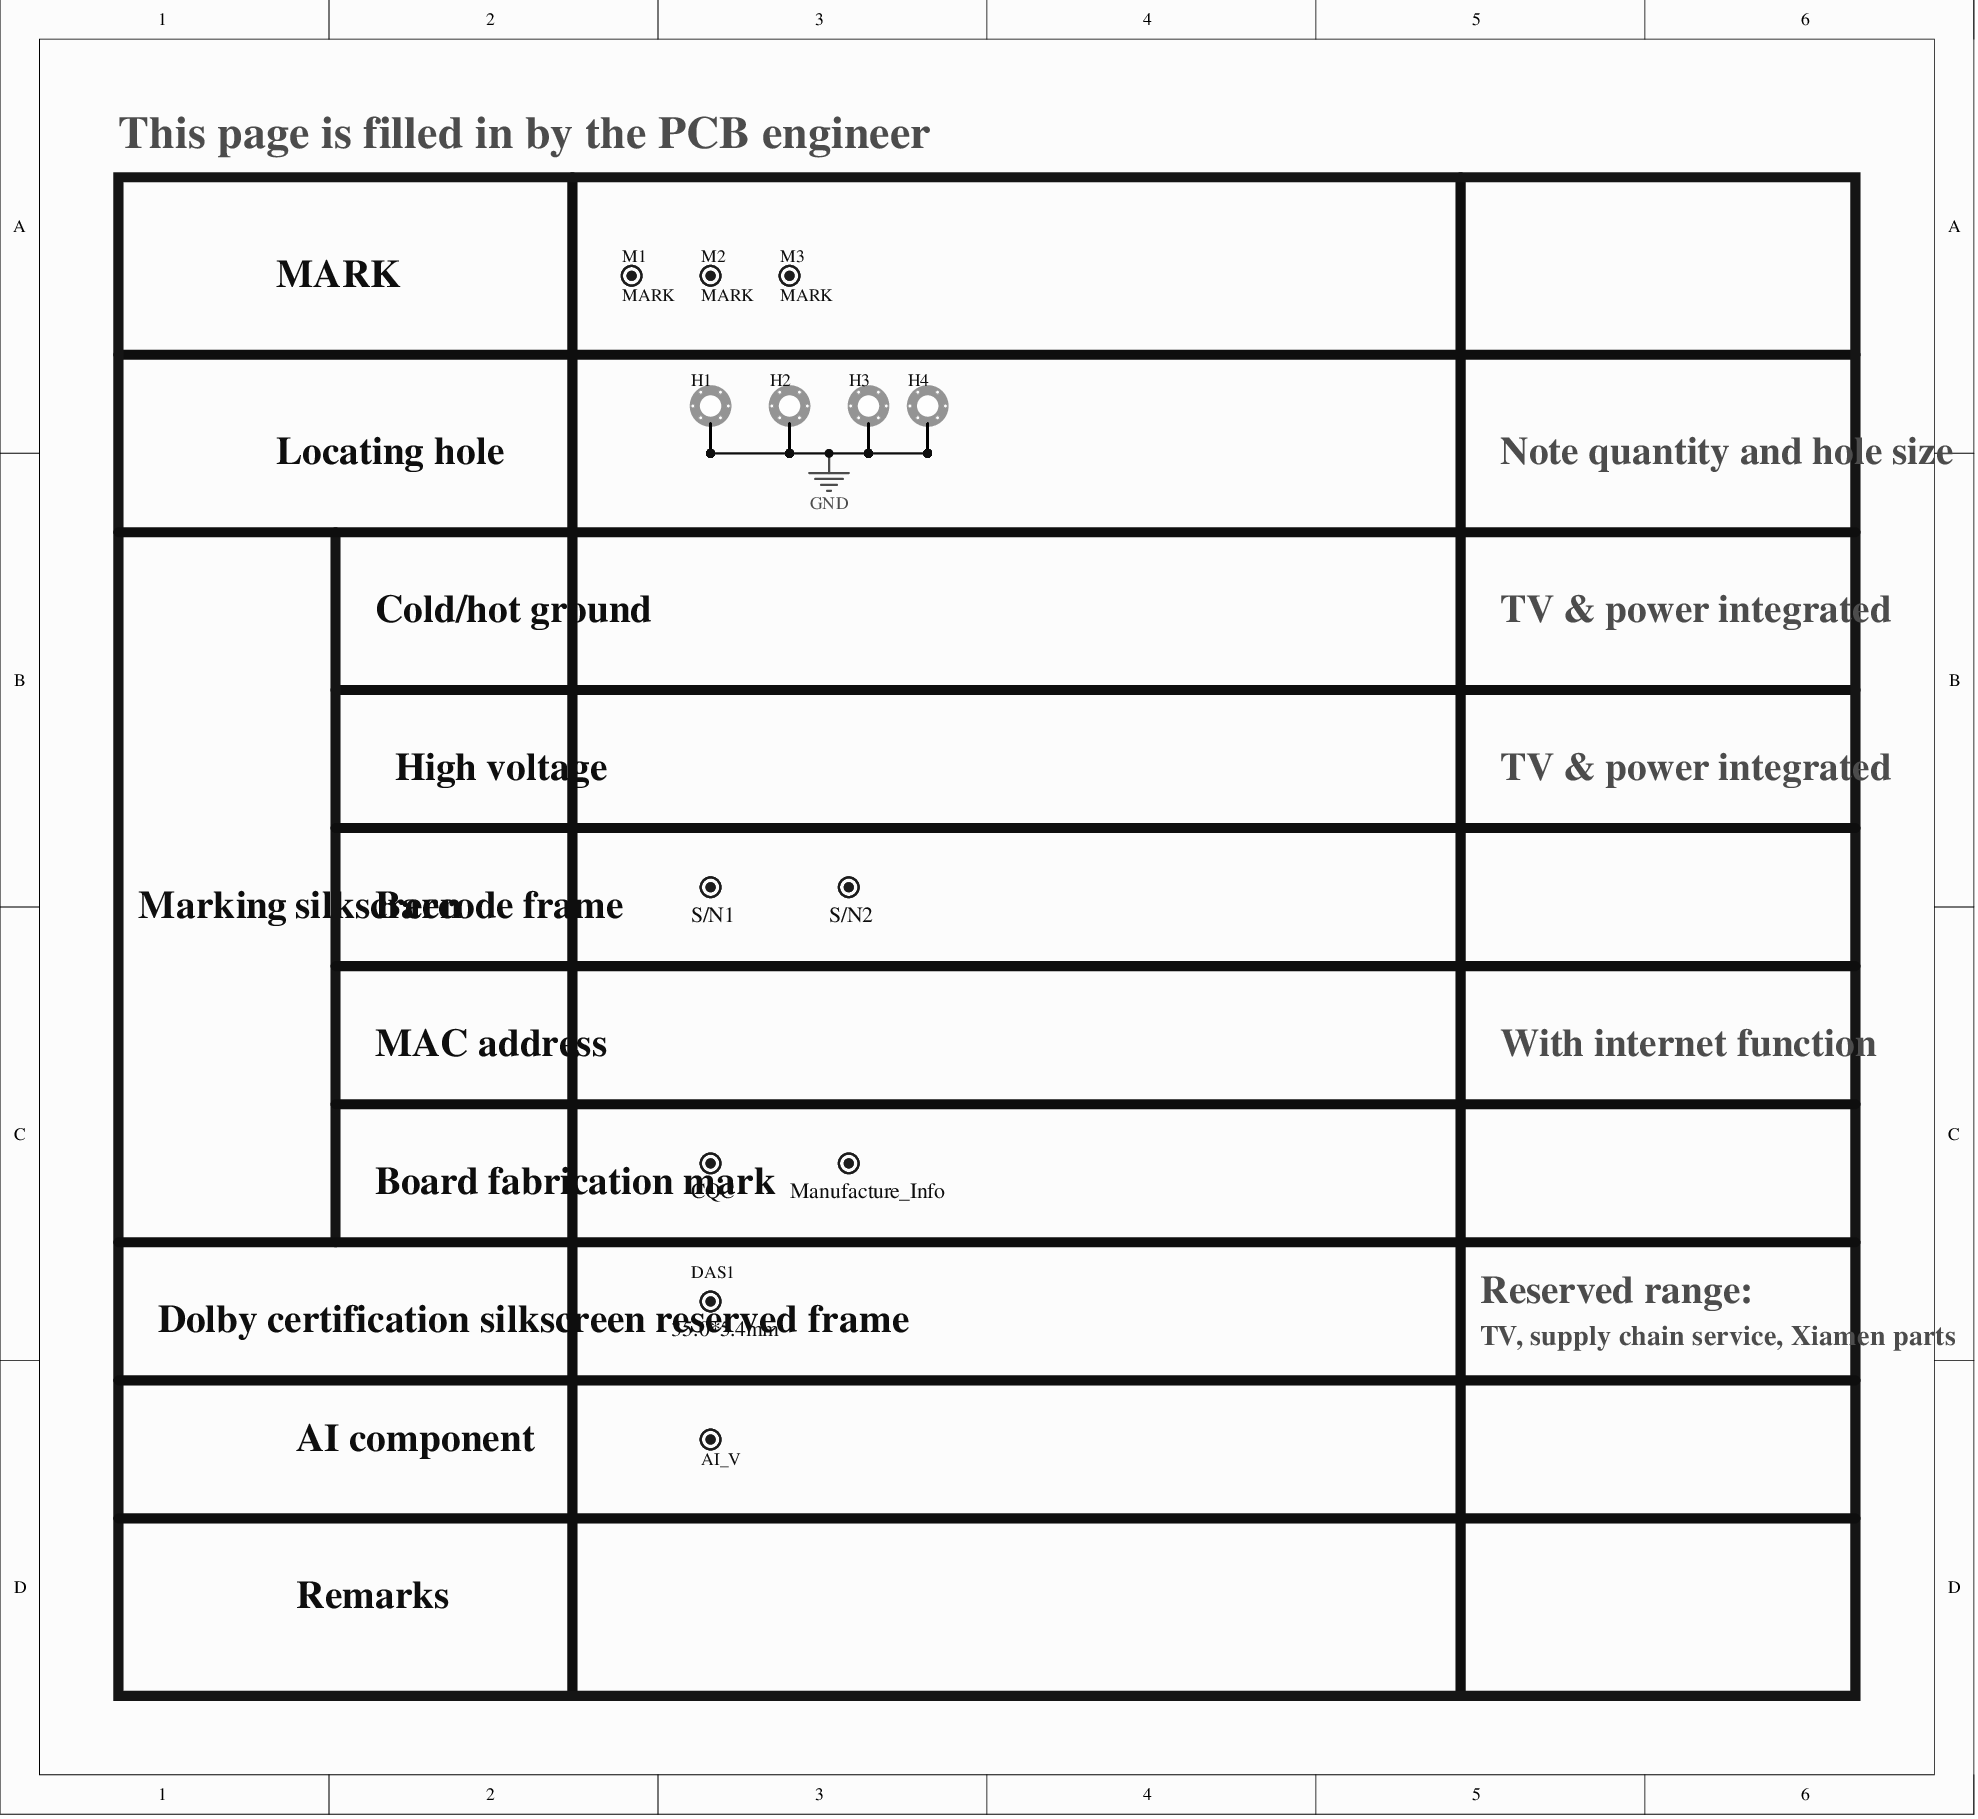
[diagram p0: MISC105950-31.SchDoc]
# Altium project MISC105950-48.PrjPCB (part 1 of 8)
13 sheets, 541 parts. Net scope: global (net labels, ports and power ports of the same name join across sheets).
Sheets:
  MISC105950-31.SchDoc
  MISC105950-32.SchDoc
  MISC105950-34.SchDoc
  MISC105950-35.SchDoc
  MISC105950-36.SchDoc
  MISC105950-37.SchDoc
  MISC105950-38.SchDoc
  MISC105950-39.SchDoc
  MISC105950-40.SchDoc
  MISC105950-41.SchDoc
  MISC105950-44.SchDoc
  MISC105950-42.SchDoc
  MISC105950-43.SchDoc

## Sheet MISC105950-31.SchDoc
size 254 x 233 mm

### Parts
AI_V  AI_GRIPPER_V  [AI_GRIPPER_V]  (value not drawn)
CQC  CQC  [CQC]
DAS1  35.0*5.4mm  [DOLBY_AS2]
H1  Location hole  [ASSE4.0C-3]  (value not drawn)
H2  Location hole  [ASSE4.0C-3]  (value not drawn)
H3  Location hole  [ASSE4.0C-3]  (value not drawn)
H4  Location hole  [ASSE4.0C-3]  (value not drawn)
M1  MARK  [MARK]
M2  MARK  [MARK]
M3  MARK  [MARK]
Manufacture_Info  Manufacture_Info  [Manufacture_Info]
S/N1  Barcode  [Barcode]  (value not drawn)
S/N2  Barcode  [Barcode]  (value not drawn)

### Nets
GND: H1.1 H1.2 H1.3 H1.4 H1.5 H1.6 H2.1 H2.2 H2.3 H2.4 H2.5 H2.6 H3.1 H3.2 H3.3 H3.4 H3.5 H3.6 H4.1 H4.2 H4.3 H4.4 H4.5 H4.6

### Notes on the sheet
- This page is filled in by the PCB engineer
- MARK
- Locating hole
- Note quantity and hole size
- Cold/hot ground
- TV & power integrated
- High voltage
- Marking silkscreen
- Barcode frame
- MAC address
- With internet function
- (near CQC) Board fabrication mark
- (near DAS1) Dolby certification silkscreen reserved frame
- Reserved range:
- TV, supply chain service, Xiamen parts
- AI component
- Remarks

### Library data of the parts
DAS1 = DOLBY_AS2
H1-H4 = Location hole-D
M1-M3 = MARK-D

## Sheet MISC105950-32.SchDoc
size 254 x 322 mm
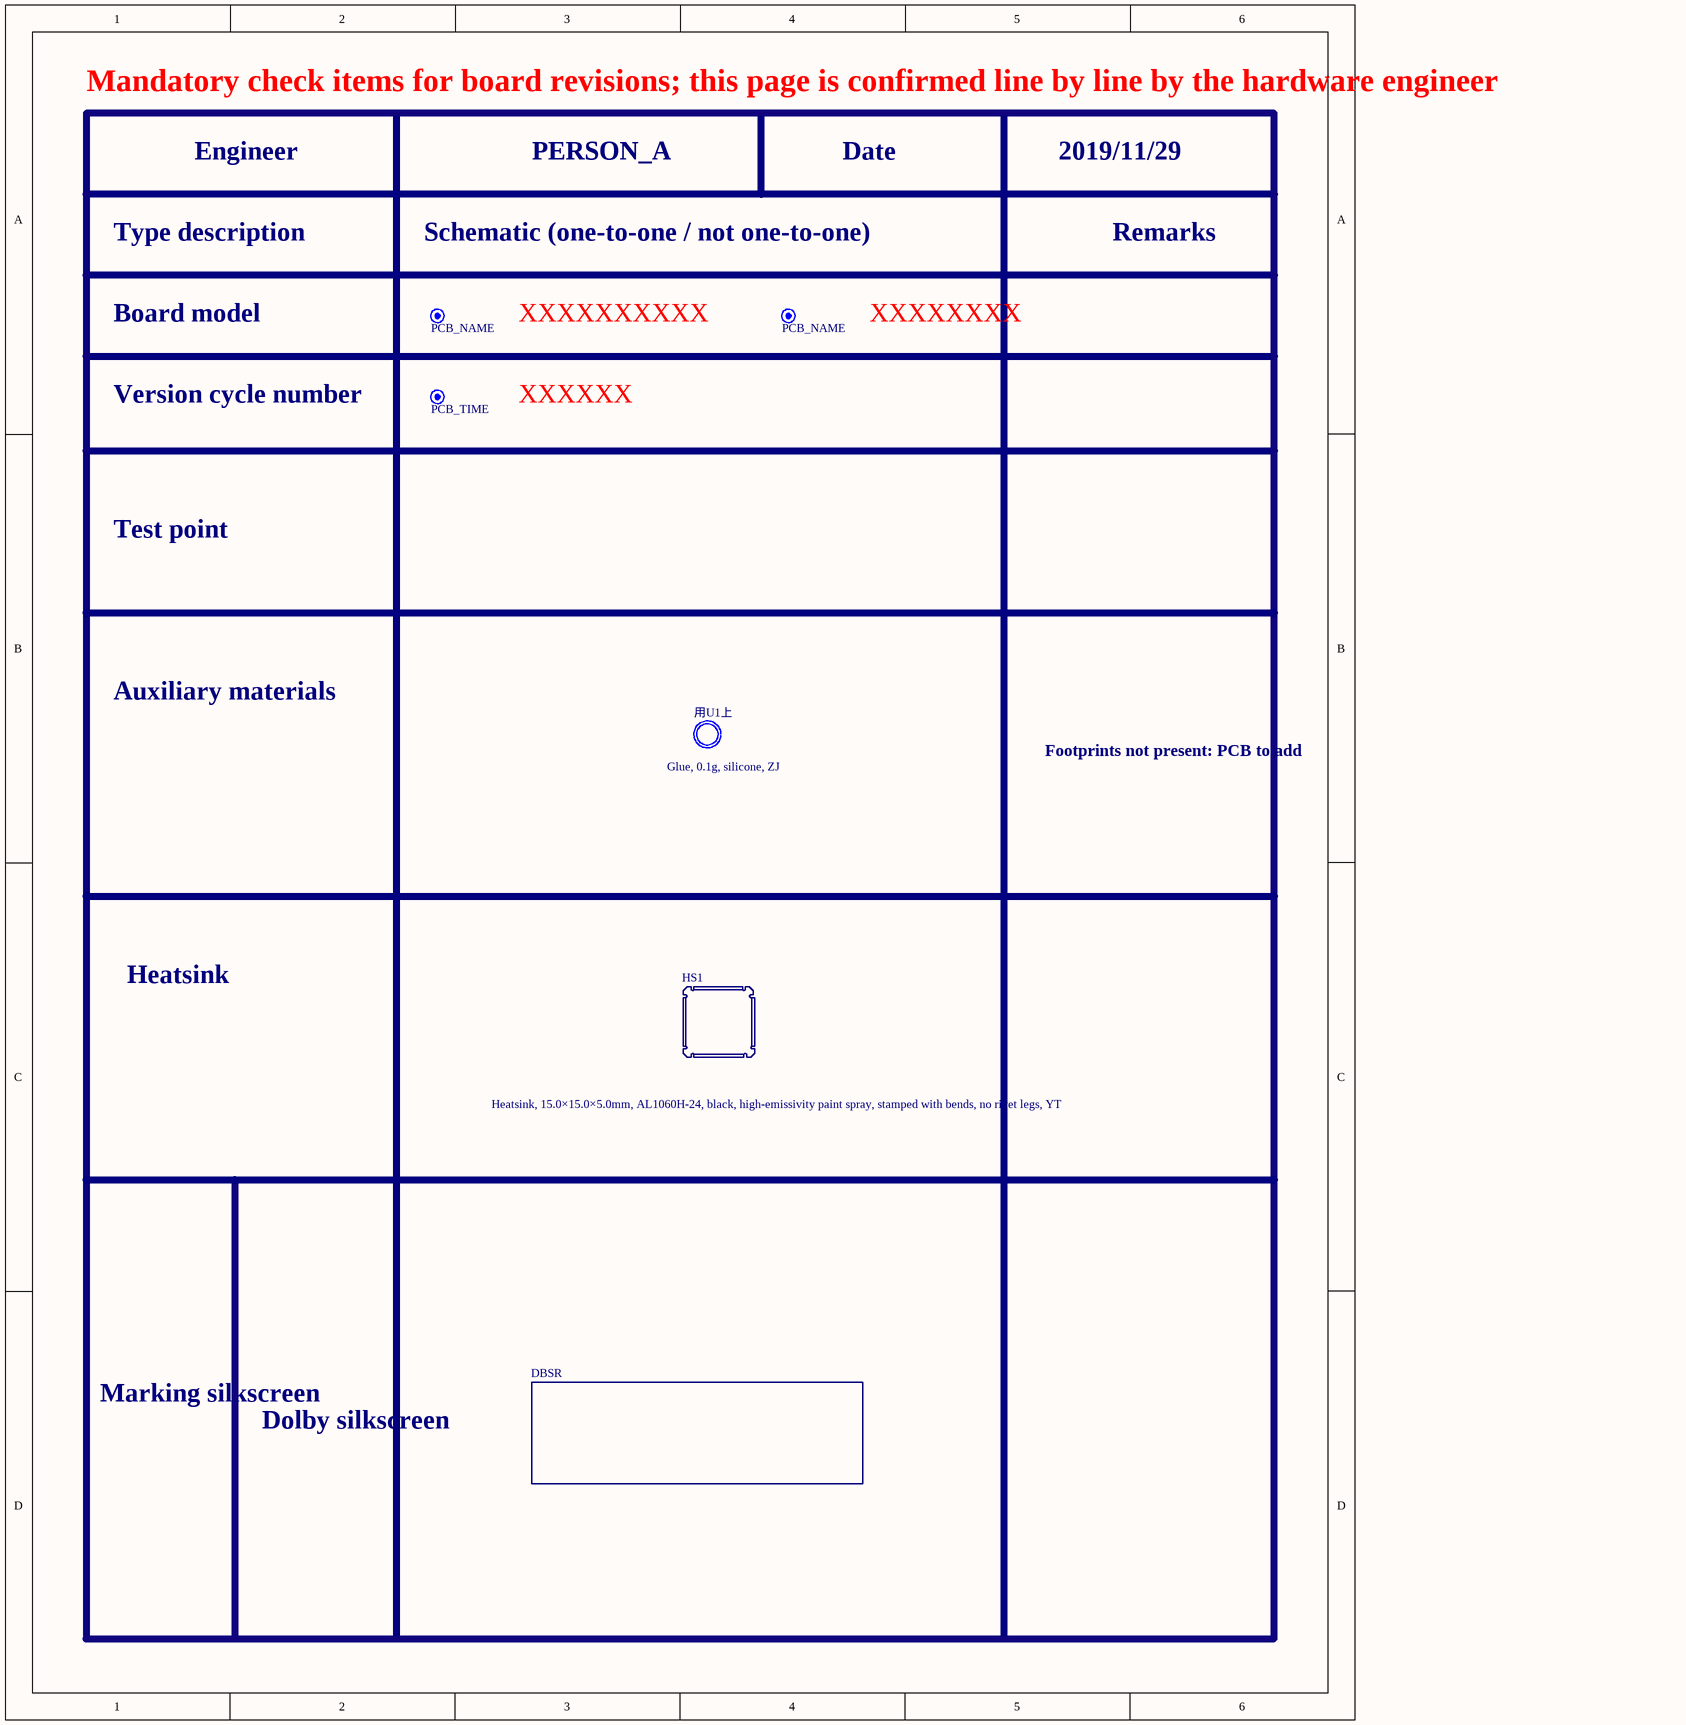
[diagram p1: MISC105950-32.SchDoc]

### Parts
DBSR  NO DOLBY  [NO DOLBY-SILK]  (value not drawn)
HS1  Heatsink, 15.0×15.0×5.0mm, AL1060H-24, black, high-emissivity paint spray, stamped with bends, no rivet legs, YT  [HS(15X15X5)-S]
XXXXXX  PCB_TIME  [PCB_TIME]
XXXXXXXX  PCB_NAME  [PCB_NAME]
XXXXXXXXXX  PCB_NAME  [PCB_NAME]
用U1上  Glue, 0.1g, silicone, ZJ  [Heat-Shrinkable Tube]

### Notes on the sheet
- Mandatory check items for board revisions; this page is confirmed line by line by the hardware engineer
- Engineer
- PERSON_A
- Date
- 2019/11/29
- Type description
- Schematic (one-to-one / not one-to-one)
- Remarks
- Board model
- Version cycle number
- Test point
- Auxiliary materials
- Footprints not present: PCB to add
- Heatsink
- Marking silkscreen
- Dolby silkscreen

### Library data of the parts
HS1 = 004.040.0008928-D: Heatsink, 15.0×15.0×5.0mm, AL1060H-24, black, high-emissivity paint spray, stamped with bends, no rivet legs, YT-D
用U1上 = Φ12mm×12mm-黑色-125度(UL认证)-D